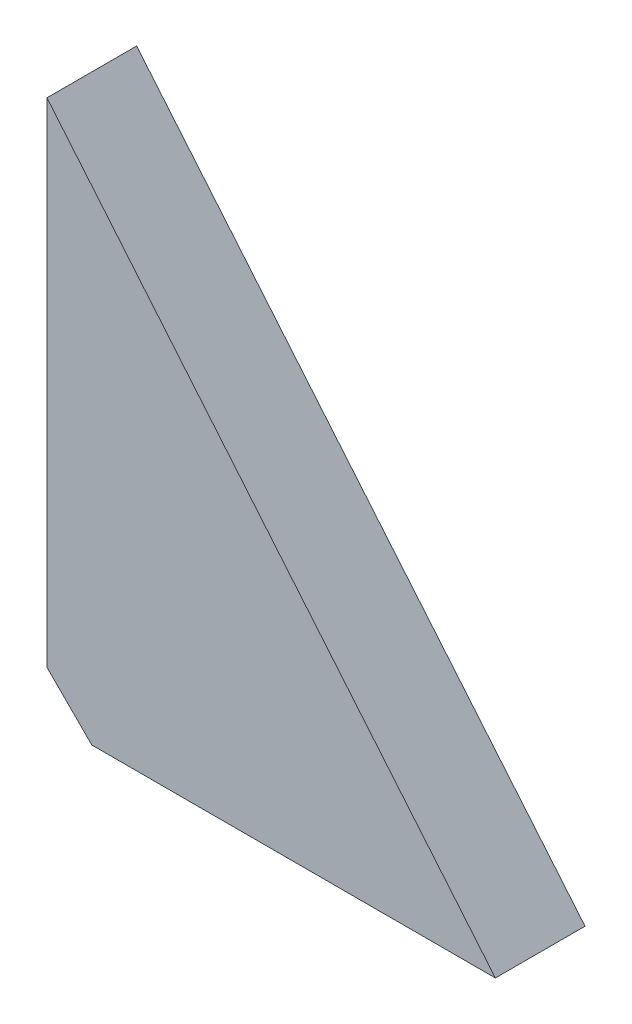
SolidWorks part; units mm, degrees
material "Q235B"
ref_plane "Front Plane" through (0, 0, 0) normal (0, 0, 1) x (1, 0, 0)
ref_plane "Top Plane" through (0, 0, 0) normal (0, 1, 0) x (1, 0, 0)
ref_plane "Right Plane" through (0, 0, 0) normal (1, 0, 0) x (0, 0, -1)
sketch "Sketch1" plane through (0, 0, 0) normal (0, 0, 1) x (1, 0, 0)
  line L0 (0, 0) -> (0, 60)
  line L1 (0, 60) -> (50, 0)
  line L2 (50, 0) -> (0, 0)
  dimension "D1" = 50
  dimension "D2" = 60
extrude "Boss-Extrude1" add sketch "Sketch1" along normal mid plane 10
chamfer "Chamfer1" distance 5 angle 45 1 edges at (0, 0, 0)
